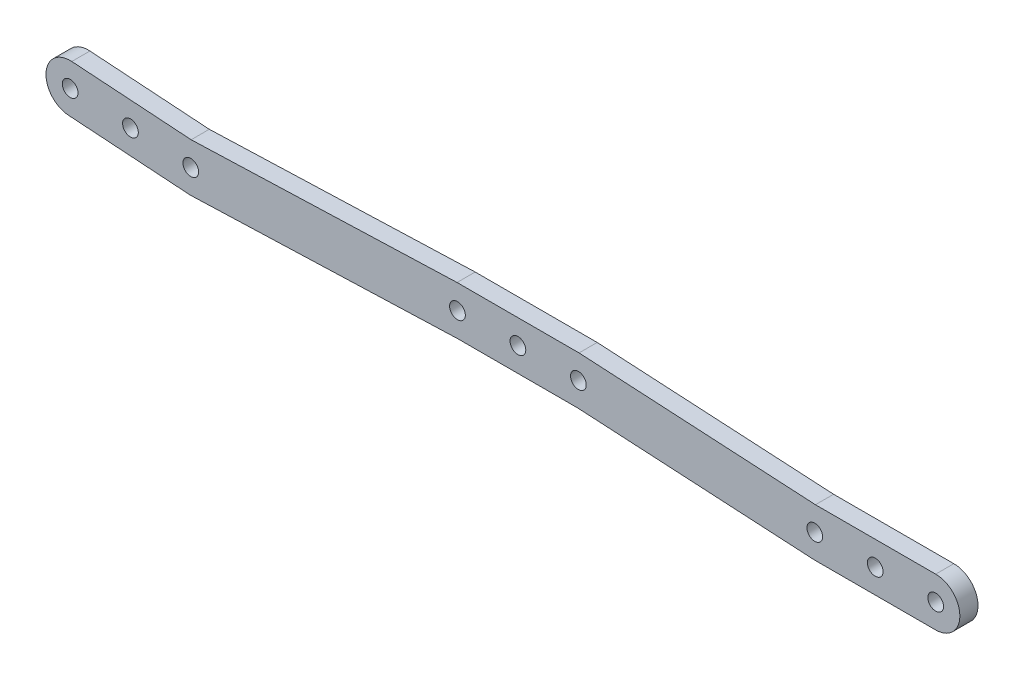
from build123d import *

# Parameters (mm, degrees)
SKETCH3_R           = 1.3
SKETCH3_R_2         = 1.299999997
SKETCH3_R_3         = 1.299999994
SKETCH3_R_4         = 1.299999992
BOSS_EXTRUDE4_DEPTH = 3


with BuildPart() as part:
    # Sketch3 → Boss-Extrude4 (new body)
    with BuildSketch(Plane.XY):
        with BuildLine():
            Line((52.490961286, -7.932397294), (42.490961286, -7.932397294))
            Line((42.490961286, -7.932397294), (32.603090799, -7.932397294))
            Line((32.603090799, -7.932397294), (-6.503485734, -5.738172333))
            Line((-6.503485734, -5.738172333), (-16.615615248, -5.738172333))
            Line((-16.615615248, -5.738172333), (-26.685781884, -5.738172333))
            Line((-26.685781884, -5.738172333), (-70.669528111, -7.281743071))
            Line((-70.669528111, -7.281743071), (-80.441339321, -6.619135373))
            Line((-80.441339321, -6.619135373), (-90.418428622, -5.942608164))
            ThreePointArc((-90.418428622, -5.942608164), (-94.679875227, -9.662833001), (-90.95965039, -13.924279606))
            Line((-90.95965039, -13.924279606), (-80.982561088, -14.600806815))
            Line((-80.982561088, -14.600806815), (-70.800193694, -15.291253536))
            Line((-70.800193694, -15.291253536), (-26.545448611, -13.738172333))
            Line((-26.545448611, -13.738172333), (-16.615615248, -13.738172333))
            Line((-16.615615248, -13.738172333), (-6.727744762, -13.738172333))
            Line((-6.727744762, -13.738172333), (32.378831772, -15.932397294))
            Line((32.378831772, -15.932397294), (42.490961286, -15.932397294))
            Line((42.490961286, -15.932397294), (52.490961286, -15.932397294))
            ThreePointArc((52.490961286, -15.932397294), (56.490961286, -11.932397294), (52.490961286, -7.932397294))
        make_face()
        with Locations((-90.689039506, -9.933443885)):
            Circle(SKETCH3_R, mode=Mode.SUBTRACT)
        with Locations((-70.734860903, -11.286498303)):
            Circle(SKETCH3_R, mode=Mode.SUBTRACT)
        with Locations((-80.711950204, -10.609971094)):
            Circle(SKETCH3_R, mode=Mode.SUBTRACT)
        with Locations((-26.615615248, -9.738172333)):
            Circle(SKETCH3_R, mode=Mode.SUBTRACT)
        with Locations((-16.615615248, -9.738172333)):
            Circle(SKETCH3_R_2, mode=Mode.SUBTRACT)
        with Locations((-6.615615248, -9.738172333)):
            Circle(SKETCH3_R_3, mode=Mode.SUBTRACT)
        with Locations((32.490961286, -11.932397294)):
            Circle(SKETCH3_R_3, mode=Mode.SUBTRACT)
        with Locations((42.490961286, -11.932397294)):
            Circle(SKETCH3_R_4, mode=Mode.SUBTRACT)
        with Locations((52.490961286, -11.932397294)):
            Circle(SKETCH3_R, mode=Mode.SUBTRACT)
    extrude(amount=BOSS_EXTRUDE4_DEPTH)


solid = part.part
